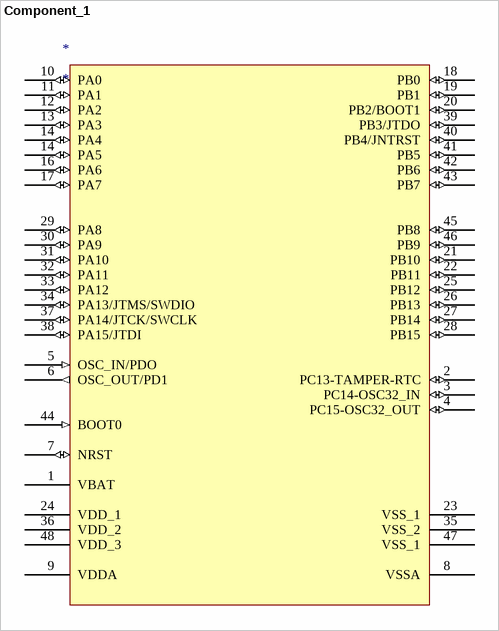
[diagram p0: symbol Component_1]
# Altium schematic symbol library MISC80722-8.SchLib: 1 symbol
Pins are listed as number, name and electrical type; pins without a type are passive.


## Component_1
designator *
pins: 1 VBAT, 2 PC13-TAMPER-RTC (io), 3 PC14-OSC32_IN (io), 4 PC15-OSC32_OUT (io), 5 OSC_IN/PDO (in), 6 OSC_OUT/PD1 (out), 7 NRST (io), 8 VSSA, 9 VDDA, 10 PA0 (io), 11 PA1 (io), 12 PA2 (io), 13 PA3 (io), 14 PA5 (io), 14 PA4 (io), 16 PA6 (io), 17 PA7 (io), 18 PB0 (io), 19 PB1 (io), 20 PB2/BOOT1 (io), 21 PB10 (io), 22 PB11 (io), 23 VSS_1, 24 VDD_1, 25 PB12 (io), 26 PB13 (io), 27 PB14 (io), 28 PB15 (io), 29 PA8 (io), 30 PA9 (io), 31 PA10 (io), 32 PA11 (io), 33 PA12 (io), 34 PA13/JTMS/SWDIO (io), 35 VSS_2, 36 VDD_2, 37 PA14/JTCK/SWCLK (io), 38 PA15/JTDI (io), 39 PB3/JTDO (io), 40 PB4/JNTRST (io), 41 PB5 (io), 42 PB6 (io), 43 PB7 (io), 44 BOOT0 (in), 45 PB8 (io), 46 PB9 (io), 47 VSS_1, 48 VDD_3